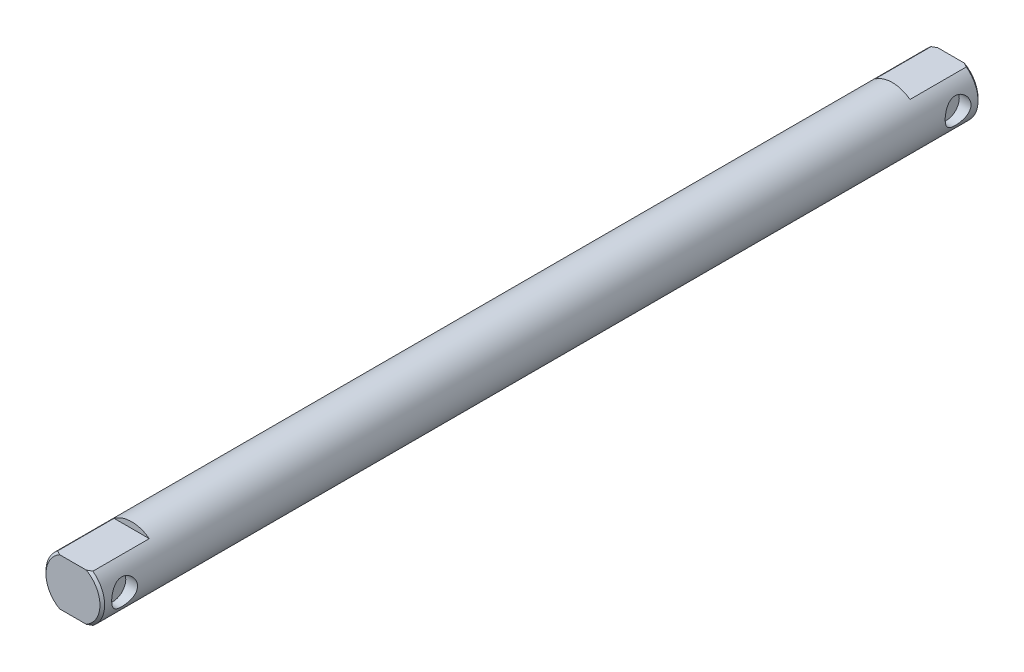
from build123d import *

# Parameters (mm, degrees)
SKETCH_1_R          = 12.5
EXTRUDE_1_DEPTH     = 187
CHAMFER_1_SIZE      = 1
SKETCH_2_W          = 25
SKETCH_2_H          = 25
CUT_EXTRUDE_1_DEPTH = 2.5
SKETCH_3_R          = 5.5
CUT_EXTRUDE_2_DEPTH = 5


with BuildPart() as part:
    # 草图1 → 凸台-拉伸1 (new, symmetric)
    with BuildSketch(Plane.XY):
        Circle(SKETCH_1_R)
    extrude(amount=EXTRUDE_1_DEPTH, both=True)

    # 倒角1
    chamfer_1_edges = [part.edges().sort_by_distance(p)[0] for p in [
        (-12.5, 0, -187),
        (-12.5, 0, 187),
    ]]
    chamfer(chamfer_1_edges, length=CHAMFER_1_SIZE)

    # 草图2 → 切除-拉伸1 (cut)
    with BuildSketch(Plane(origin=(0, 12.5, 0), x_dir=(1, 0, 0), z_dir=(0, 1, 0))):
        with Locations((0, -174.5)):
            Rectangle(SKETCH_2_W, SKETCH_2_H)
        with Locations((0, 174.5)):
            Rectangle(SKETCH_2_W, SKETCH_2_H)
    cut_extrude_1 = extrude(amount=-CUT_EXTRUDE_1_DEPTH, mode=Mode.SUBTRACT)

    # 镜向1: 切除-拉伸1 across plane
    add(cut_extrude_1.mirror(Plane.ZX), mode=Mode.SUBTRACT)

    # 草图3 → 切除-拉伸2 (cut)
    with BuildSketch(Plane(origin=(12.5, 0, 0), x_dir=(0, 0, -1), z_dir=(1, 0, 0))):
        with Locations((-177.5, 0)):
            Circle(SKETCH_3_R)
        with Locations((177.5, 0)):
            Circle(SKETCH_3_R)
    extrude(amount=-CUT_EXTRUDE_2_DEPTH, mode=Mode.SUBTRACT)


solid = part.part
